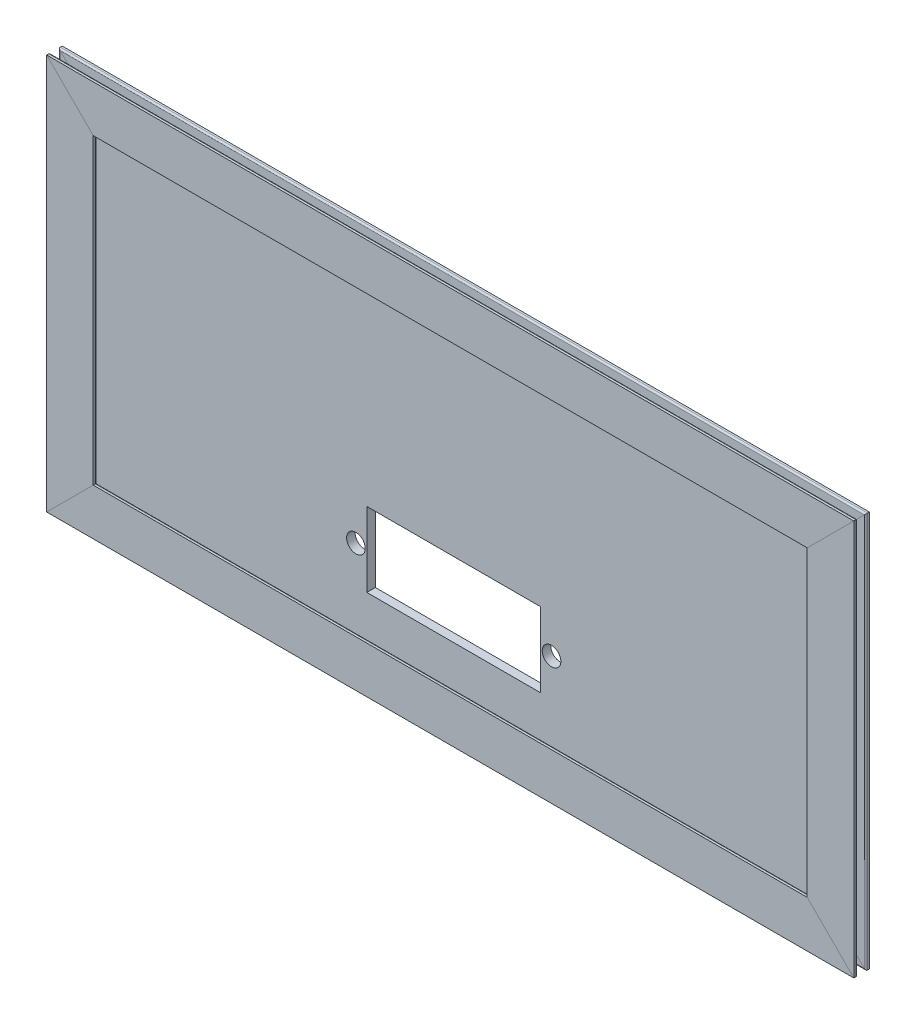
SolidWorks part; units mm, degrees
ref_plane "Front Plane" through (0, 0, 0) normal (0, 0, 1) x (1, 0, 0)
ref_plane "Top Plane" through (0, 0, 0) normal (0, 1, 0) x (1, 0, 0)
ref_plane "Right Plane" through (0, 0, 0) normal (1, 0, 0) x (0, 0, -1)
sketch "Sketch 1" plane through (0, 0, 0) normal (0, 0, 1) x (1, 0, 0)
  line L1 (-245, -112.5) -> (245, -112.5)
  line L2 (-245, -112.5) -> (-245, 112.5)
  line L3 (-245, 112.5) -> (245, 112.5)
  line L4 (245, -112.5) -> (245, 112.5)
  line L5 (-245, -112.5) -> (245, 112.5) construction
  line L6 (-245, 112.5) -> (245, -112.5) construction
  point P0 (0, 0)
  dimension "D1" = 490
  dimension "D2" = 225
other "Aluminium profile 20 X 20 X 2(1)"
ref_plane "Plane1" through (-245, 112.5, 0) normal (1, 0, 0) x (0, 1, 0)
sketch "Sketch1" plane through (-245, 112.5, 0) normal (1, 0, 0) x (0, 1, 0)
  line L0 (-3.1, -2.2) -> (3.1, -2.2)
  line L1 (3.1, -2.2) -> (3.1, 2.2)
  line L2 (3.1, 2.2) -> (-3.1, 2.2)
  line L3 (-3.1, 2.2) -> (-3.1, -2.2)
  line L4 (4.5, 2.75) -> (14, 2.75)
  line L5 (4.5, -2.75) -> (4.5, 2.75)
  line L6 (14, -2.75) -> (4.5, -2.75)
  line L7 (15, -5) -> (15, -3.75)
  line L8 (-15, -5) -> (15, -5)
  line L9 (-15, -3.75) -> (-15, -5)
  line L10 (-4.5, -2.75) -> (-14, -2.75)
  line L11 (-4.5, 2.75) -> (-4.5, -2.75)
  line L12 (-14, 2.75) -> (-4.5, 2.75)
  line L13 (-15, 5) -> (-15, 3.75)
  line L14 (15, 5) -> (-15, 5)
  line L15 (15, 3.75) -> (15, 5)
  arc A0 (15, -3.75) -> (14, -2.75) centre (14, -3.75) ccw
  arc A1 (-14, -2.75) -> (-15, -3.75) centre (-14, -3.75) ccw
  arc A2 (-15, 3.75) -> (-14, 2.75) centre (-14, 3.75) ccw
  arc A3 (14, 2.75) -> (15, 3.75) centre (14, 3.75) ccw
  point P24 (0, 0)
sketch "Sketch3" plane through (0, 0, -2.75) normal (0, 0, 1) x (1, 0, 0)
  line L1 (-231, 98.5) -> (231, 98.5)
  line L2 (-231, 98.5) -> (-231, -98.5)
  line L3 (-231, -98.5) -> (231, -98.5)
  line L4 (231, 98.5) -> (231, -98.5)
extrude "Boss-Extrude1" add sketch "Sketch3" along normal up to surface (5.5 mm away) separate body up to face at (0, -103.25, 2.75)
sketch "Sketch4" plane through (0, 0, -2.75) normal (0, 0, -1) x (-1, 0, 0)
  line L0 (230, -97.5) -> (-230, -97.5) construction
  line L1 (56, -71.5) -> (-56, -71.5)
  line L2 (56, -71.5) -> (56, -23.5)
  line L3 (56, -23.5) -> (-56, -23.5)
  line L4 (-56, -71.5) -> (-56, -23.5)
  line L5 (56, -71.5) -> (-56, -23.5) construction
  line L6 (56, -23.5) -> (-56, -71.5) construction
  line L7 (-63, -47.5) -> (63, -47.5) construction
  line L8 (0, 0) -> (0, -47.5) construction
  circle A0 centre (-63, -47.5) radius 6
  circle A1 centre (63, -47.5) radius 6
  point P0 (0, -47.5)
  point P15 (0, -47.5)
  dimension "D5" = 12
  dimension "D1" = 50
  dimension "D2" = 112
  dimension "D3" = 48
  dimension "D4" = 126
extrude "Cut-Extrude1" cut sketch "Sketch4" against normal through all
